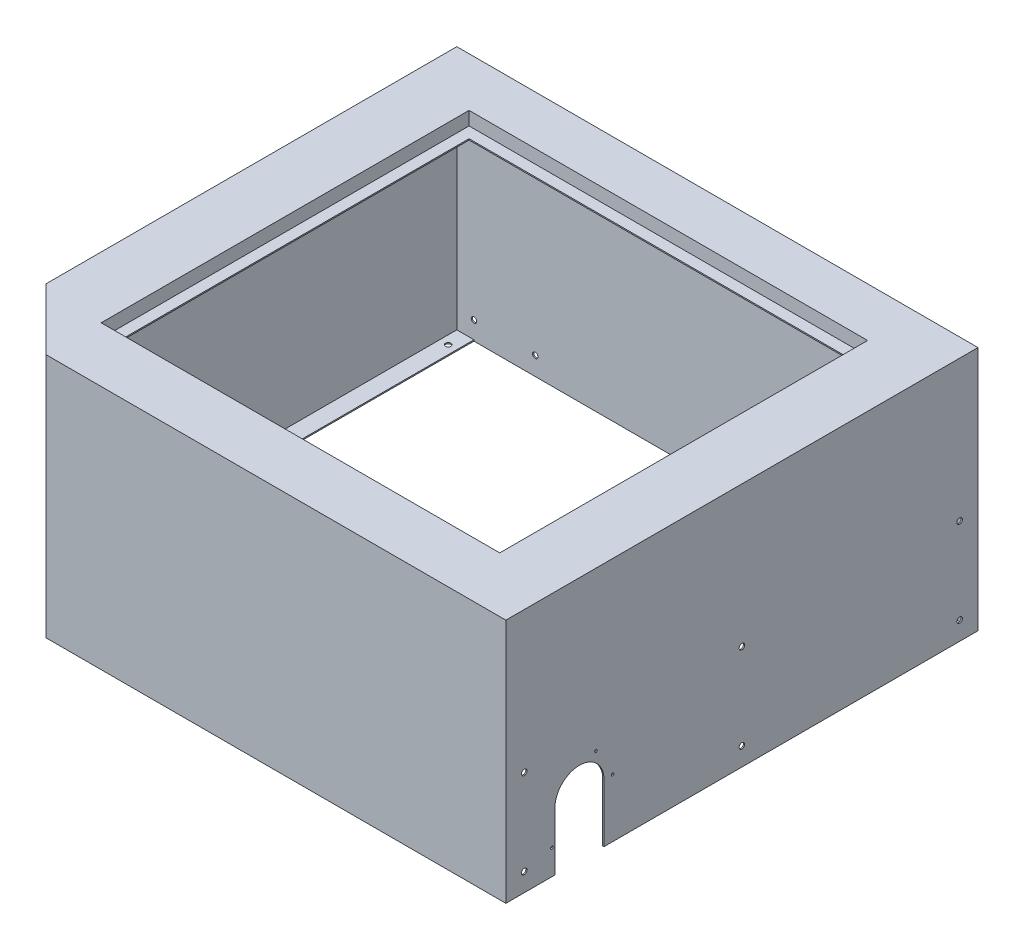
SolidWorks part; units mm, degrees
ref_plane "前视" through (0, 0, 0) normal (0, 0, 1) x (1, 0, 0)
ref_plane "上视" through (0, 0, 0) normal (0, 1, 0) x (1, 0, 0)
ref_plane "右视" through (0, 0, 0) normal (1, 0, 0) x (0, 0, -1)
sketch "草图1" plane through (0, 0, 0) normal (0, 1, 0) x (1, 0, 0)
  line L0 (0, 0) -> (51.5592, 0) construction
  line L1 (0, 0) -> (0, 51.0384) construction
  line L2 (-425, 380) -> (-425, -290)
  line L3 (-425, 380) -> (425, 380)
  line L4 (425, -390) -> (-325, -390)
  line L5 (-325, -390) -> (-425, -290)
  line L6 (425, 380) -> (425, -390)
  dimension "D1" = 850
  dimension "D2" = 770
  dimension "D3" = 380
  dimension "D4" = 425
  dimension "D5" = 670
  dimension "D6" = 750
extrude "凸台-拉伸1" add sketch "草图1" against normal blind 400
shell "抽壳1" thickness 2
sketch "草图3" plane through (0, 0, 0) normal (0, 1, 0) x (1, 0, 0)
  line L0 (0, 0) -> (0, 297.6632) construction
  line L1 (-325, 300) -> (325, 300)
  line L2 (-325, 300) -> (-325, -300)
  line L3 (-325, -300) -> (325, -300)
  line L4 (325, 300) -> (325, -300)
  line L5 (0, 0) -> (500.2151, 0) construction
  dimension "D1" = 650
  dimension "D2" = 600
  dimension "D3" = 300
  dimension "D4" = 325
extrude "切除-拉伸1" cut sketch "草图3" against normal blind 2
sketch "草图4" plane through (0, 0, 0) normal (0, 1, 0) x (1, 0, 0)
  line L0 (0, 0) -> (505.1565, 0) construction
  line L1 (-327, 302) -> (327, 302)
  line L2 (-327, 302) -> (-327, -302)
  line L3 (-327, -302) -> (327, -302)
  line L4 (327, 302) -> (327, -302)
  line L5 (0, 0) -> (0, 413.4211) construction
  line L7 (-325, 300) -> (325, 300)
  line L8 (-325, 300) -> (-325, -300)
  line L9 (-325, -300) -> (325, -300)
  line L10 (325, 300) -> (325, -300)
  dimension "D1" = 2
  dimension "D2" = 2
  dimension "D3" = 2
  dimension "D4" = 2
extrude "凸台-拉伸2" add sketch "草图4" against normal blind 24
sketch "草图5" plane through (0, -24, 0) normal (0, -1, 0) x (1, 0, 0)
  line L0 (307, 282) -> (307, -282)
  line L1 (-327, 302) -> (327, 302)
  line L2 (-327, 302) -> (-327, -302)
  line L3 (-327, -302) -> (327, -302)
  line L4 (327, 302) -> (327, -302)
  line L5 (-307, -282) -> (307, -282)
  line L7 (-307, 282) -> (-307, -282)
  line L8 (-307, 282) -> (307, 282)
  dimension "D1" = 20
extrude "凸台-拉伸3" add sketch "草图5" against normal blind 2
sketch "草图6" plane through (0, -400, 0) normal (0, -1, 0) x (1, 0, 0)
  line L0 (-425, 290) -> (-325, 390)
  line L1 (-325, 390) -> (425, 390)
  line L2 (425, 390) -> (425, 360)
  line L3 (425, 390) -> (425, -380) construction
  line L4 (425, 360) -> (-312.5736, 360)
  line L5 (-425, 290) -> (-403.7868, 268.7868)
  line L6 (-403.7868, 268.7868) -> (-312.5736, 360)
  dimension "D1" = 30
  dimension "D2" = 30
extrude "凸台-拉伸4" add sketch "草图6" against normal blind 2
sketch "草图7" plane through (425, 0, 0) normal (1, 0, 0) x (0, 0, -1)
  line L0 (-310, -400) -> (-310, -305)
  line L1 (-390, -400) -> (380, -400) construction
  line L2 (-270, -400) -> (-270, -157.943) construction
  line L3 (-230, -305) -> (-230, -400)
  line L4 (-230, -400) -> (-310, -400)
  line L7 (-390, -400) -> (-390, 0) construction
  arc A0 (-230, -305) -> (-310, -305) centre (-270, -305) ccw
  dimension "D2" = 40
  dimension "D1" = 80
  dimension "D3" = 80
  dimension "D4" = 95
extrude "切除-拉伸2" cut sketch "草图7" against normal blind 2
ref_plane "基准面1" through (-150, 0, 0) normal (-1, 0, 0) x (0, 0, 1)
sketch "草图10" plane through (-423, 0, 0) normal (1, 0, 0) x (0, 0, -1)
  line L1 (378, -400) -> (-288, -400)
  line L2 (378, -400) -> (378, -398)
  line L3 (378, -398) -> (-288, -398)
  line L4 (-288, -400) -> (-288, -398)
extrude "凸台-拉伸7" add sketch "草图10" along normal blind 28
sketch "草图12" plane through (0, -398, 0) normal (0, 1, 0) x (1, 0, 0)
  line L0 (-425, 380) -> (-425, -290) construction
  line L6 (425, 380) -> (-425, 380) construction
  line L7 (425, -390) -> (425, -310) construction
  line L9 (-318.3726, -374) -> (423, -374)
  line L10 (-409, -283.3726) -> (-318.3726, -374)
  line L11 (-409, 378) -> (-409, -283.3726)
  line L12 (-318.3726, -374) -> (423, -374) construction
  line L13 (-409, -283.3726) -> (-318.3726, -374) construction
  line L14 (-409, 378) -> (-409, -283.3726) construction
  circle A0 centre (-409, 350) radius 4.5
  circle A1 centre (-363.6863, -328.6863) radius 4.5
  circle A2 centre (-85, -374) radius 4.5
  circle A3 centre (395, -374) radius 4.5
  circle A4 centre (-409, -90) radius 4.5
  circle A5 centre (-25, -374) radius 4.5
  circle A6 centre (-409, -150) radius 4.5
  circle A7 centre (23, -374) radius 4.5
  circle A8 centre (123, -374) radius 4.5
  dimension "D2" = 9
  dimension "D3" = 30
  dimension "D4" = 9
  dimension "D5" = 9
  dimension "D6" = 470
  dimension "D7" = 9
  dimension "D8" = 9
  dimension "D9" = 30
  dimension "D10" = 450
  dimension "D11" = 9
  dimension "D12" = 60
  dimension "D13" = 9
  dimension "D14" = 60
  dimension "D15" = 9
  dimension "D16" = 9
  dimension "D17" = 100
  dimension "D18" = 448
  dimension "D1" = 14
extrude "切除-拉伸3" cut sketch "草图12" against normal blind 10
sketch "草图13" plane through (0, 0, -378) normal (0, 0, 1) x (1, 0, 0)
  line L0 (0, -400) -> (0, 140.1404) construction
  line L1 (-325, -400) -> (425, -400) construction
  line L4 (-425, -400) -> (-425, 0) construction
  line L5 (-295, -370) -> (295, -370) construction
  line L6 (-295, -370) -> (-295, -30) construction
  line L7 (-295, -30) -> (295, -30) construction
  line L8 (295, -370) -> (295, -30) construction
  line L10 (-325, 0) -> (425, 0) construction
  line L11 (-395, 53.3886) -> (-395, -473.8169) construction
  line L12 (-295, -30) -> (-518.1633, -30) construction
  line L13 (-295, -370) -> (-510.1982, -370) construction
  circle A0 centre (0, -30) radius 4.5
  circle A1 centre (-295, -30) radius 4.5
  circle A2 centre (0, -370) radius 4.5
  circle A3 centre (-295, -370) radius 4.5
  circle A4 centre (-395, -30) radius 4.5
  circle A5 centre (-395, -370) radius 4.5
  circle A6 centre (295, -30) radius 4.5
  circle A7 centre (295, -370) radius 4.5
  circle A8 centre (395, -370) radius 4.5
  circle A9 centre (395, -30) radius 4.5
  dimension "D6" = 9
  dimension "D7" = 9
  dimension "D8" = 9
  dimension "D9" = 9
  dimension "D10" = 9
  dimension "D11" = 9
  dimension "D1" = 130
  dimension "D3" = 30
  dimension "D4" = 30
  dimension "D5" = 30
extrude "切除-拉伸4" cut sketch "草图13" against normal blind 10
sketch "草图14" plane through (425, 0, 0) normal (1, 0, 0) x (0, 0, -1)
  line L1 (-390, -400) -> (-390, 0) construction
  line L2 (-360, -370) -> (350, -370) construction
  line L3 (-360, -370) -> (-360, -230) construction
  line L4 (-360, -230) -> (350, -230) construction
  line L5 (350, -370) -> (350, -230) construction
  line L6 (380, -400) -> (380, 0) construction
  line L7 (-230, -400) -> (380, -400) construction
  line L8 (-5, -230) -> (-5, -475.4977) construction
  circle A0 centre (-360, -230) radius 4.5
  circle A1 centre (-360, -370) radius 4.5
  circle A2 centre (-5, -230) radius 4.5
  circle A3 centre (-5, -370) radius 4.5
  circle A4 centre (350, -370) radius 4.5
  circle A5 centre (350, -230) radius 4.5
  dimension "D5" = 9
  dimension "D6" = 9
  dimension "D7" = 9
  dimension "D8" = 9
  dimension "D1" = 30
  dimension "D2" = 30
  dimension "D3" = 30
  dimension "D4" = 140
extrude "切除-拉伸5" cut sketch "草图14" against normal blind 10
hole_wizard "M5 螺纹孔1" positions "草图16" profile "草图15" tap size "M5" standard "GB"
sketch "草图16" plane through (425, 0, 0) normal (1, 0, 0) x (0, 0, -1)
  line L0 (-270, -359) -> (-380.0405, -359) construction
  line L2 (-243, -258.2346) -> (-270, -305) construction
  line L3 (-270, -305) -> (-270, -227.2108) construction
  circle A0 centre (-270, -305) radius 54 construction
  point P0 (-243, -258.2346)
  point P1 (-216, -305)
  point P3 (-315, -359)
  dimension "D1" = 108
  dimension "D2" = 45
  dimension "D3" = 30
sketch "草图15" plane through (425, -258.2346, 243) normal (0, 1, 0) x (0, 0, -1)
  line L0 (0, 0) -> (0, 4.2618)
  line L1 (0, 4.2618) -> (2.1, 3)
  line L2 (2.1, 3) -> (2.1, 0)
  line L5 (2.1, 0) -> (0, 0)
  line L10 (0, 4.2618) -> (-2.1, 3) construction
  line L11 (0, -6.35) -> (0, 107.95) construction
  dimension "螺纹孔钻头直径" = 4.2
  dimension "螺纹孔钻头深度" = 3
  dimension "导头角度" = 118
cosmetic thread "孔螺蚊线1" parameters "D1"=2, "D2"=5
cosmetic thread "孔螺蚊线2" parameters "D1"=2, "D2"=5
cosmetic thread "孔螺蚊线3" parameters "D1"=2, "D2"=5
